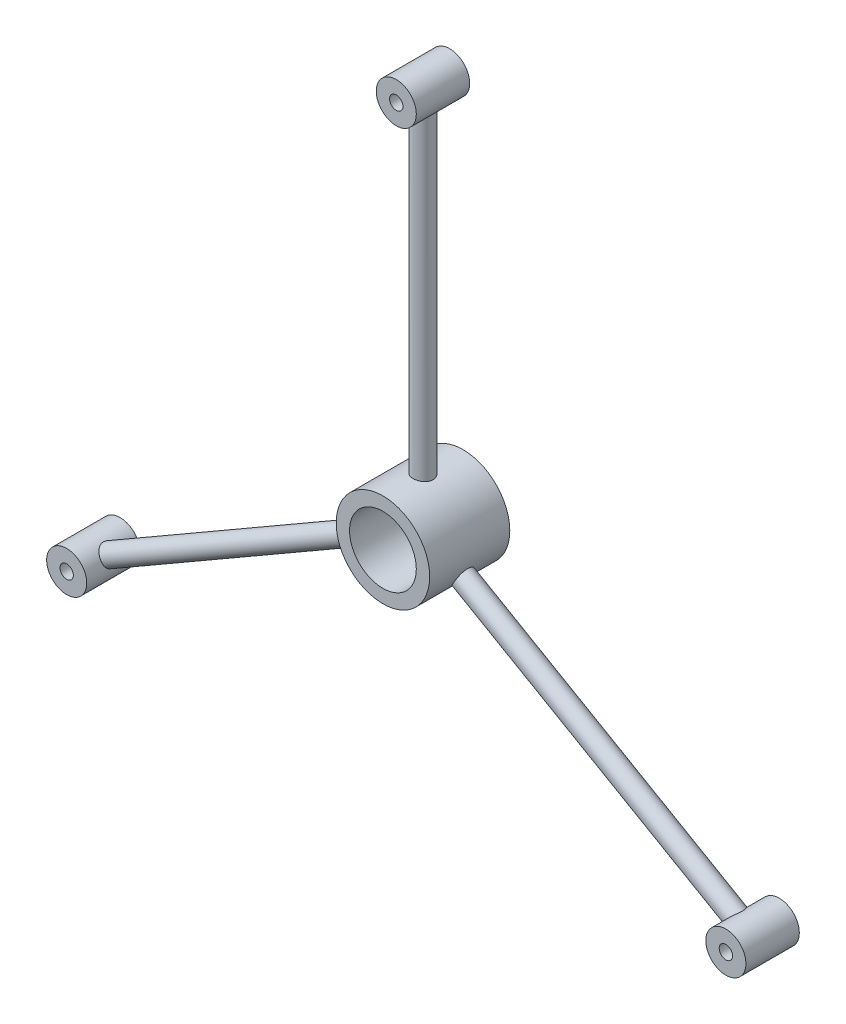
SolidWorks part; units mm, degrees
ref_plane "Front Plane" through (0, 0, 0) normal (0, 0, 1) x (1, 0, 0)
ref_plane "Top Plane" through (0, 0, 0) normal (0, 1, 0) x (1, 0, 0)
ref_plane "Right Plane" through (0, 0, 0) normal (1, 0, 0) x (0, 0, -1)
sketch "Sketch1" plane through (0, 0, 0) normal (0, 0, 1) x (1, 0, 0)
  circle A0 centre (0, 0) radius 25
  circle A1 centre (0, 0) radius 35
  dimension "D1" = 50
  dimension "D2" = 10
extrude "Boss-Extrude1" add sketch "Sketch1" along normal mid plane 60
ref_plane "Plane1" through (0, 25, 0) normal (0, 1, 0) x (1, 0, 0)
sketch "Sketch3" plane through (0, 25, 0) normal (0, 1, 0) x (1, 0, 0)
  line L0 (0, 30) -> (0, -30) construction
  line L2 (25, 30) -> (-25, 30) construction
  line L3 (-35, -30) -> (35, -30) construction
  circle A0 centre (0, 0) radius 7.5
  dimension "D1" = 15
extrude "Boss-Extrude2" add sketch "Sketch3" along normal blind 251 separate body
sketch "Sketch4" plane through (0, 0, 0) normal (0, 0, 1) x (1, 0, 0)
  line L0 (0, 285) -> (0, 0) construction
  line L2 (7.5, 276) -> (-7.5, 276) construction
  circle A0 centre (0, 285) radius 15
  circle A1 centre (0, 285) radius 5
  dimension "D1" = 10
  dimension "D2" = 30
  dimension "D3" = 6
extrude "Boss-Extrude3" add sketch "Sketch4" along normal mid plane 40
pattern_circular "CirPattern3" count 3 over 360 about axis through (0, 0, 0) along (0, 0, 1) of "Boss-Extrude2", "Boss-Extrude3"
equation "\"A\"= \"代号代码\""
equation "\"B\"= \"名称代码\""
